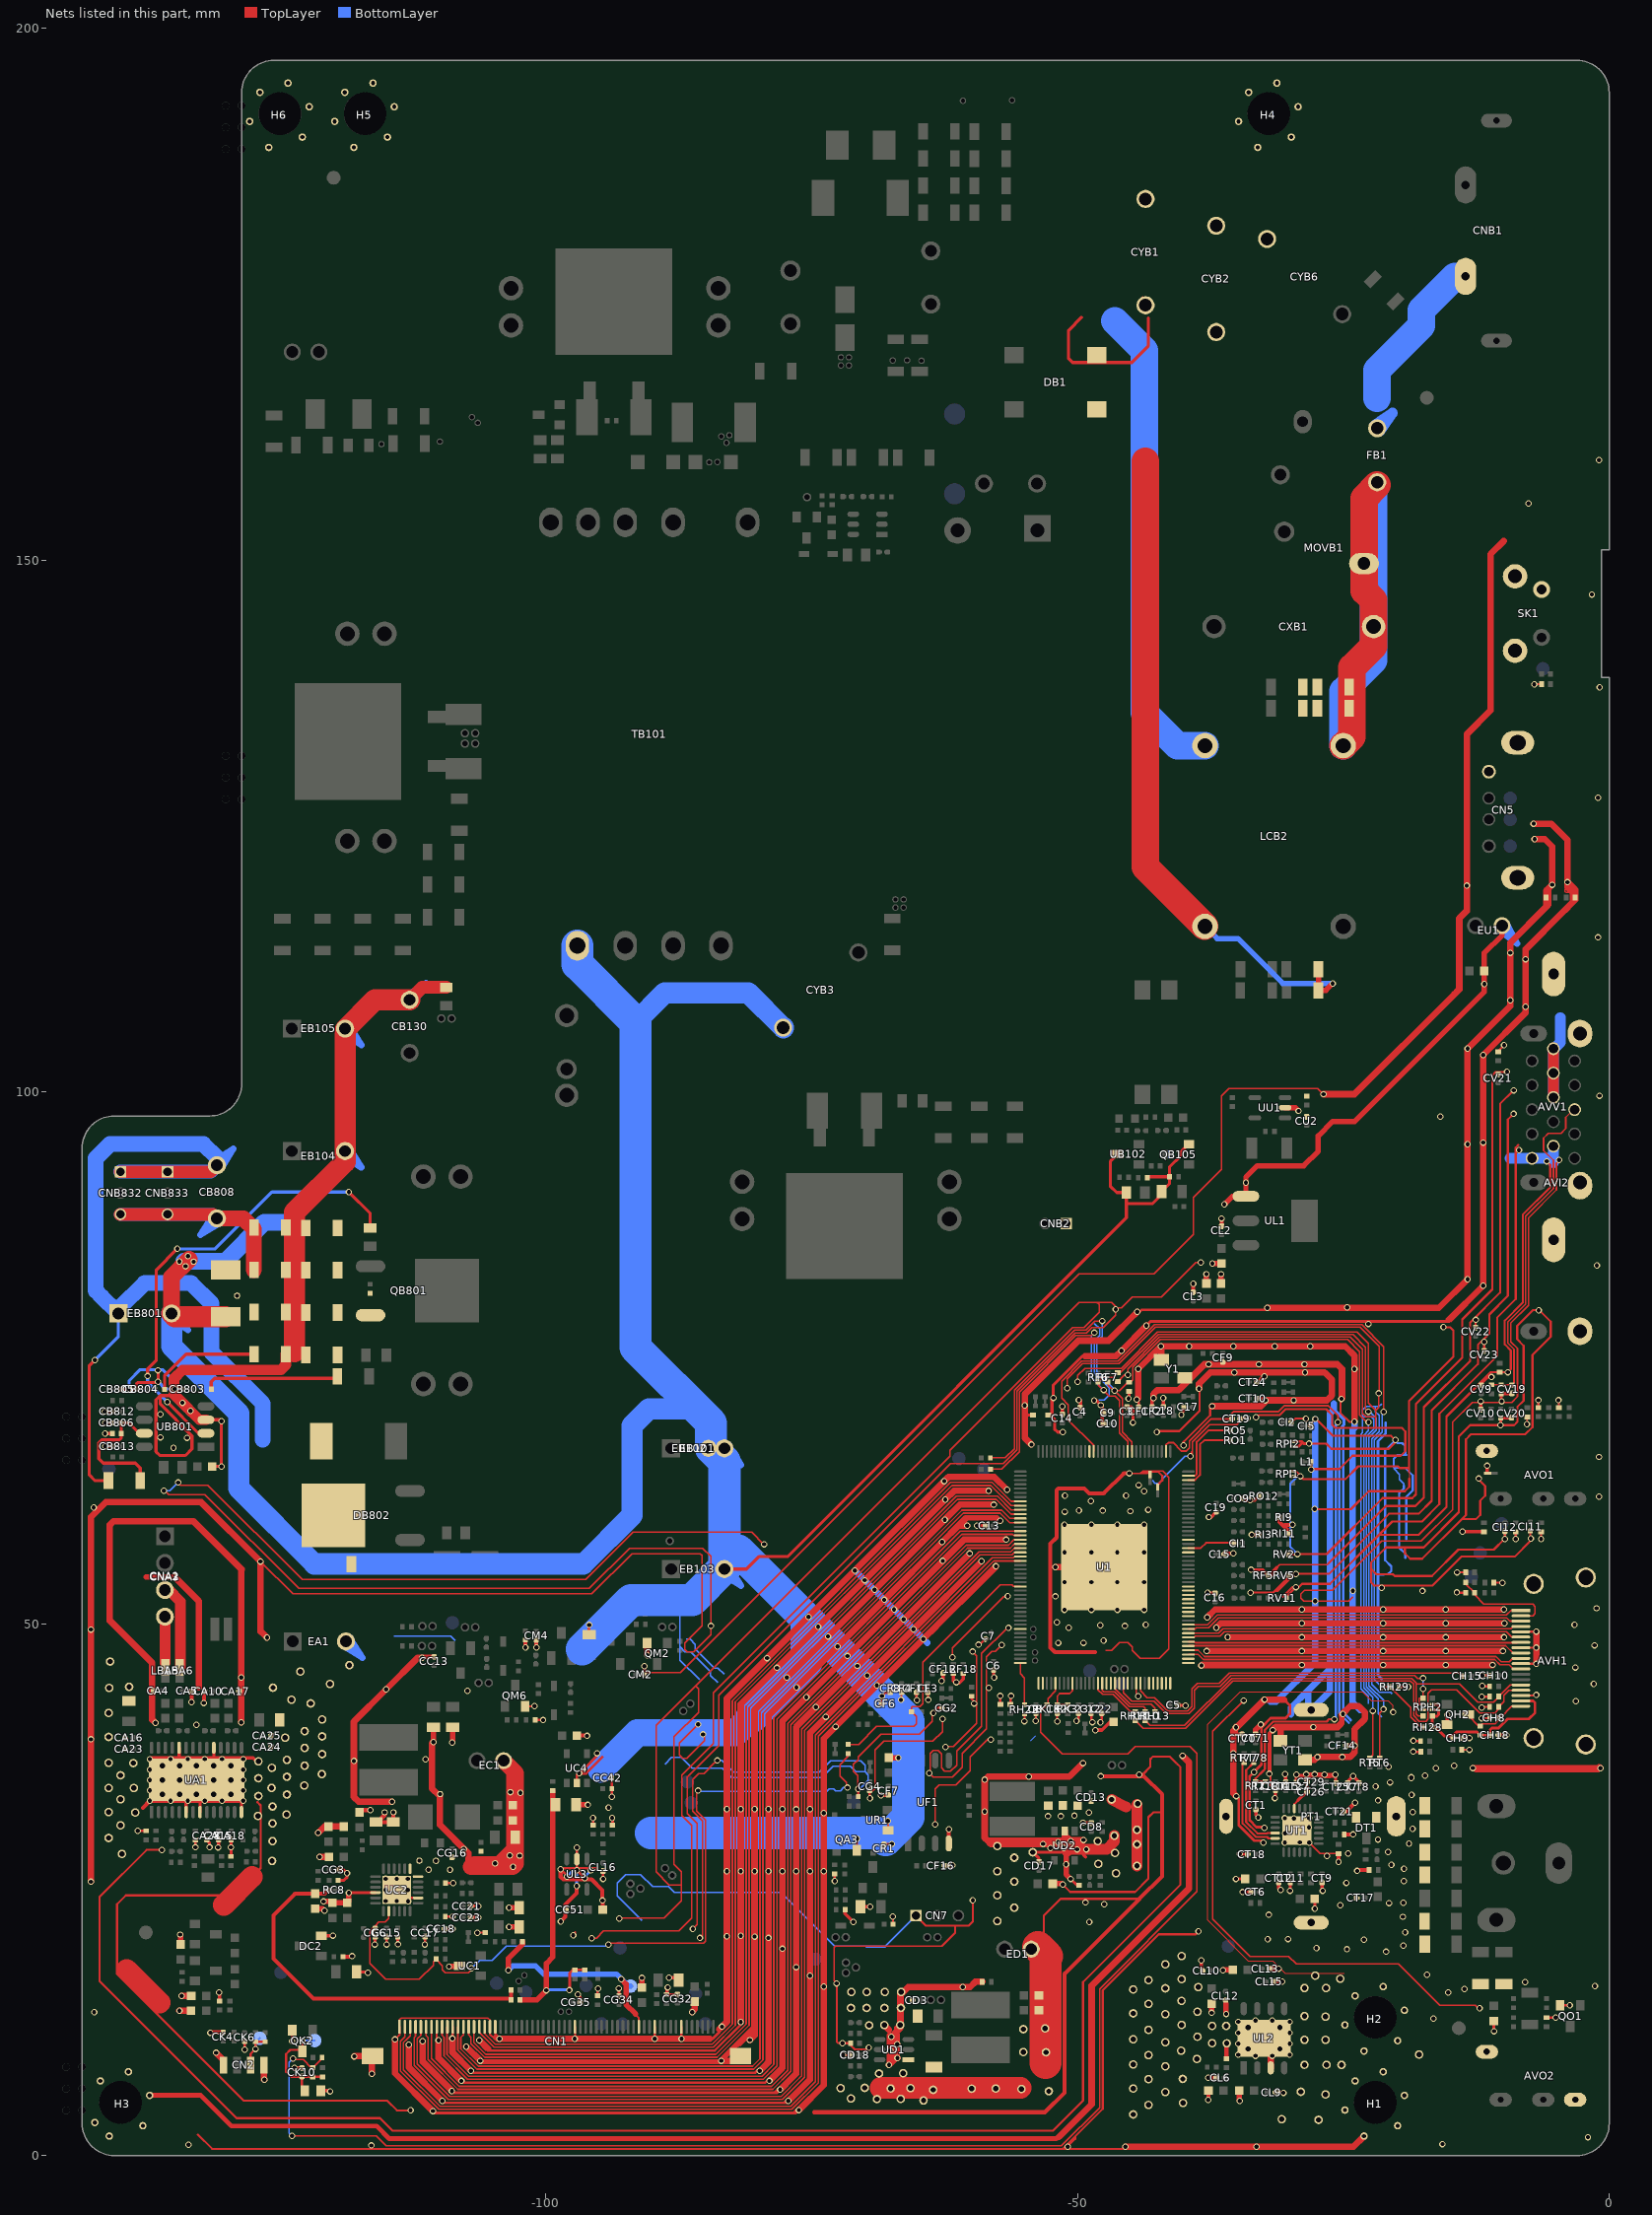
[diagram p0: the nets of this part, all layers, seen from the top]
# Altium PCB MISC86383-9.PcbDoc (part 12 of 18)
Units mm, origin at the board's own origin, x right, y up, seen from the top; angles counter-clockwise.
Board outline 143.6 x 197 mm, 2 copper layers (TopLayer, BottomLayer), stack 1.571 mm thick; 743 components, 401 nets, 2996 pads, 1077 vias.
Unrouted connection lines stored in the file: 4.

## Via types
v1: diameter 0.6, hole 0.4, TopLayer to BottomLayer, tented both sides, 993 vias
v2: diameter 0.6, hole 0.4, TopLayer to BottomLayer, 65 vias
v3: diameter 0.7, hole 0.5, TopLayer to BottomLayer, tented both sides, 15 vias
v4: diameter 0.8, hole 0.5, TopLayer to BottomLayer, tented both sides, 4 vias

## Nets (pads, with @x,y where several pads share a name; then routed paths per layer and width w, separated by ;. In a path a pad name is that pad's centre, name@x,y a point inside that pad or via, vN(x,y) a via of type N, cw(c..) or ccw(c..) an arc to the next point about the centre after c; other vN are vias at no path point) (continued)
GND: (continued)
  other v1: -116.412,0.947 -133.613,1.003 -15.673,1.074 -1.998,1.72 -33.252,9.371 -31.671,9.371 -34.884,9.476 -30.039,9.476 -34.884,10.508 -30.039,10.508 -34.884,11.539 -30.039,11.539 -34.884,12.571 -30.039,12.571 -33.252,12.677 -31.671,12.677 -16.523,12.874 -142.467,13.479 -15.146,15.329 -13.603,15.641 -1.344,15.939 -7.902,16.311 -17.141,16.988 -20.982,19.156 -24.662,19.388 -27.529,19.513 -19.363,19.748 -23.061,20.283 -32.119,20.335 -30.201,20.354 -19.19,20.979 -103.454,21.483 -48.895,21.971 -19.396,22.445 -32.013,22.636 -103.454,23.312 -47.498,23.622 -20.705,23.735 -49.258,23.792 -19.355,23.774 -112.943,23.91 -115.057,23.933 -114.012,23.927 -115.06,24.971 -112.968,24.975 -24.711,25.641 -19.317,25.819 -115.055,26.016 -114.016,26.02 -112.971,26.014 -82.969,26.73 -81.668,26.73 -80.368,26.738 -79.066,26.724 -77.765,26.736 -76.464,26.72 -75.164,26.732 -73.863,26.721 -19.293,26.964 -20.485,27.33 -25.448,27.612 -26.527,28.158 -24.559,28.399 -20.788,28.53 -52.527,28.905 -18.821,29.337 -30.509,29.42 -29.08,29.445 -21.742,29.719 -30.484,30.29 -28.235,30.85 -29.64,31.695 -30.509,31.72 -28.21,31.72 -52.781,31.902 -51.562,31.902 -50.292,31.953 -48.92,32.258 -18.476,32.296 -76.464,32.553 -81.668,32.563 -80.368,32.572 -79.066,32.557 -77.765,32.57 -75.164,32.565 -137.238,33.362 -135.287,33.368 -133.661,33.368 -132.061,33.368 -130.461,33.368 -21.739,33.39 -18.583,33.919 -137.238,34.339 -128.452,34.339 -21.968,34.717 -20.597,35.092 -137.238,35.316 -128.452,35.316 -18.607,35.499 -18.606,35.566 -17.324,35.719 -137.238,36.293 -128.452,36.293 -16.293,36.415 -20.736,36.565 -14.575,36.637 -111.316,37.254 -135.287,37.275 -133.661,37.275 -132.061,37.275 -130.461,37.275 -128.452,37.27 -35.343,37.81 -72.747,40.329 -132.85,40.498 -73.659,41.256 -74.587,42.167 -3.144,42.729 -75.495,43.098 -107.355,43.692 -76.424,44.01 -68.874,44.196 -1.445,44.34 -77.334,44.94 -69.785,45.124 -78.26,45.854 -3.173,45.892 -70.714,46.035 -79.18,46.773 -71.622,46.966 -72.55,47.877 -1.385,47.977 -51.816,48.209 -49.428,48.209 -47.549,48.412 -73.461,48.808 -50.815,49.641 -74.387,49.721 -45.532,49.793 -47.869,49.869 -43.576,49.895 -3.256,49.916 -51.932,50.141 -75.306,50.641 -51.221,51.313 -48.69,51.313 -46.252,51.313 -43.721,51.313 -21.26,51.337 -15.354,51.337 -1.181,51.458 -52.07,52.578 -24.105,53.102 -17.568,53.086 -51.221,53.916 -48.69,53.916 -46.252,53.916 -43.721,53.916 -126.835,55.854 -51.221,56.71 -48.69,56.71 -46.252,56.71 -43.721,56.71 -6.401,57.963 -51.221,59.313 -48.69,59.313 -46.252,59.313 -43.721,59.313 -51.196,60.537 -45.018,60.588 -47.634,60.639 -49.869,60.665 -43.343,60.723 -142.515,60.934 -48.741,61.548 -0.955,61.969 -45.43,62.036 -51.179,62.056 -43.726,62.471 -44.247,63.043 -0.91,99.652 -1.05,114.538 -1.045,127.688 -0.889,138.049 -1.626,146.787 -7.569,155.346 -0.947,159.42
  other v2: -135.014,66.535 -133.731,67.488 -136.233,67.539 -134.976,68.656 -136.246,69.698 -15.875,97.688
  other v3: -136.071,33.966 -134.445,33.966 -132.845,33.966 -131.245,33.966 -129.619,33.966 -136.071,35.316 -134.445,35.316 -131.245,35.316 -129.619,35.316 -136.071,36.666 -134.445,36.666 -132.845,36.666 -131.245,36.666 -129.619,36.666
  other v4: -33.961,10.024 -30.961,10.024 -33.961,12.024 -30.961,12.024
GND1: CYB1.2 CYB2.2 CYB6.2
GREF: CN1.46 GREF.1 RG48.2 | length 20.8
  TopLayer w0.203: -91.542,13.208 -91.25,12.916 CN1.46@-91.25,12.103
  TopLayer w0.508: v1(-103.518,17.424) -103.514,17.428 -103.514,18.535 -102.191,19.859 RG48.2@-102.191,20.117 ; v1(-92.9,16.586) -92.9,16.561 -92.456,16.116 -92.456,14.211 -91.542,13.297
  BottomLayer w0.508: v1(-103.518,17.424) -103.111,17.831 -100.97,17.831 -100.186,17.047 -93.361,17.047 v1(-92.9,16.586) -92.24,15.926 GREF.1@-92.024,15.926
GVOFF: CG6.1 RG49.1 RGV1.2 UC2.8 | length 74.4
  TopLayer w0.127: CG6.1@-116.046,21.38 -116.046,21.606 ; UC2.8@-114.764,22.973 -114.764,22.302 -115.123,21.943 -115.71,21.943 -116.046,21.606 ; v1(-106.985,17.59) -106.972,17.602 -106.883,17.602 -106.94,17.545 -107.281,17.204 -109.463,17.204 -109.73,17.471 -109.73,17.857 -110.305,18.432 RG49.1@-110.305,18.466 -110.579,18.192 -110.579,17.888 -111.894,16.573 -115.077,16.573 -116.566,18.062 -116.566,21.087 -116.16,21.493 -116.046,21.606 ; v1@-94.12,19.609 v1(-94.12,19.812) ; v1@-93.916,19.964 -85.166,19.964 -84.988,20.142 -84.988,31.556 -85.809,32.377 -85.809,34.193 v1(-85.687,34.315) ; v1(-71.628,34.595) -71.742,34.595 -71.742,35.056 -72.352,35.665 -72.352,36.747 -71.564,37.534 RGV1.2@-71.564,37.802
  BottomLayer w0.127: v1(-106.985,17.59) -106.223,18.351 -105.036,18.351 -103.715,19.672 -94.259,19.672 v1(-94.12,19.812) ; v1(-85.687,34.315) -85.598,34.227 -73.566,34.227 -73.33,34.463 -72.923,34.463 -72.75,34.29 -72.301,34.29 -71.996,34.595 v1(-71.628,34.595)
GVOFF/: RG40.1 RGV1.1 U1.106 | length 26.3
  TopLayer w0.127: RGV1.1@-71.564,38.652 -70.588,38.652 -68.888,40.352 -65.387,40.352 -65.168,40.571 -65.168,41.292 -65.601,41.725 RG40.1@-65.608,41.725 -65.608,42.113 -65.51,42.211 -64.799,42.211 -64.541,42.469 -64.541,46.391 -57.274,53.659 -56.147,53.659 -56.001,53.513 U1.106@-55.371,53.513
HD1_PB: U1.27
HD1_PR: U1.30
HD1_Y: CI1.1 U1.28 | length 4.5
  TopLayer w0.178: U1.28@-39.571,57.113 -38.404,57.113 -37.91,57.607 -35.343,57.607 CI1.1@-35.307,57.571
HDMI1_DET: U1.66
HDMI1_RX0_N: U1.153
HDMI1_RX0_P: U1.154
HDMI1_RX1_N: U1.155
HDMI1_RX1_P: U1.156
HDMI1_RX2_N: U1.1@-39.571,46.313 | length 0.3
  TopLayer w0.178: U1.1@-39.571,46.313 U1.1@-39.237,46.313
HDMI1_RX2_P: U1.2
HDMI1_RXC_N: U1.151
HDMI1_RXC_P: U1.152
HDMI1_SCL: U1.126
HDMI1_SDA: U1.125
HDMI2_5V: AVH1.18 CH9.2@-14.526,39.261 CH9.2@-14.701,39.261 CH18.2@-11.046,39.54 CH18.2@-11.221,39.54 RH14.2 RH28.2 RPH2.1 RPH2.3 RPH2.5 | length 17.7
  TopLayer w0.254: RPH2.3@-16.606,41.914 -16.146,41.914 -16.04,41.808 ; RPH2.5@-16.606,42.414 -16.602,42.418 -16.091,42.418 -16.04,42.367 -16.04,41.808 ; CH9.2@-14.783,39.439 -15.509,39.439 -16.354,40.284 RH28.2@-16.644,40.284 -16.644,41.276 RPH2.1@-16.606,41.314 -16.179,41.314 -16.04,41.453 -16.04,41.808 ; CH9.2@-14.701,39.261 -14.701,39.49 -14.371,39.82 -12.44,39.82 RH14.2@-12.142,39.522 -11.239,39.522 CH18.2@-11.221,39.54 -11.195,39.566 -11.195,40.029 -11.024,40.201 -10.412,40.201 -9.557,41.055 -7.56,41.055 -6.968,41.647 -6.968,42.57 -7.148,42.75 AVH1.18@-8.3,42.75
HDMI2_DET: RH28.1 RH29.1 U1.65 | length 79.6
  TopLayer w0.127: U1.65@-48.471,66.213 -48.471,66.759 -50.848,69.136 -50.848,70.584 -51.486,71.222 -51.486,72.805 -49.598,74.693 -46.197,74.693 -42.782,78.108 -23.269,78.108 -21.193,76.032 v1@-21.193,69.954 ; v1(-21.37,44.042) -21.351,44.061 RH29.1@-20.619,44.061 -18.656,42.098 -18.656,41.258 -17.682,40.284 RH28.1@-17.494,40.284
  BottomLayer w0.127: v1(-21.37,44.042) -22.068,44.74 -22.068,67.287 -21.331,68.024 v1@-21.331,69.803
  other v1: -21.216,69.93
HDMI2_RX0_N: AVH1.9 U1.5 | length 31.3
  TopLayer w0.155: U1.5@-39.571,47.913 -39.545,47.939 -9.732,47.939 -9.043,47.25 AVH1.9@-8.57,47.25
HDMI2_RX0_P: AVH1.7 U1.6 | length 31
  TopLayer w0.155: U1.6@-39.571,48.313 -38.991,48.313 -38.899,48.221 -8.64,48.221 AVH1.7@-8.611,48.25
HDMI2_RX1_N: AVH1.6 U1.7 | length 31.1
  TopLayer w0.155: U1.7@-39.571,48.713 -39.044,48.713 -38.949,48.808 -38.945,48.808 -38.922,48.831 -36.589,48.831 -36.175,49.246 -9.667,49.246 -9.171,48.75 AVH1.6@-8.926,48.75
HDMI2_RX1_P: AVH1.4@-8.3,49.75 U1.8 | length 31.5
  TopLayer w0.155: U1.8@-39.571,49.113 -36.732,49.113 -36.317,49.528 -9.245,49.528 -9.022,49.75 AVH1.4@-8.3,49.75
HDMI2_RX2_N: AVH1.3 U1.9 | length 31.8
  TopLayer w0.155: U1.9@-39.571,49.513 -38.93,49.513 -38.812,49.631 -37.654,49.631 -36.739,50.546 -9.642,50.546 -9.346,50.25 AVH1.3@-8.3,50.25
HDMI2_RX2_P: AVH1.1 U1.10 | length 31.3
  TopLayer w0.155: U1.10@-39.571,49.913 -37.771,49.913 -36.855,50.828 -9.655,50.828 -9.233,51.25 AVH1.1@-8.775,51.25
HDMI2_RXC_N: AVH1.12 U1.3 | length 31.8
  TopLayer w0.155: U1.3@-39.571,47.113 -38.653,47.113 -38.179,46.638 -10.759,46.638 -10.267,46.146 -9.418,46.146 -9.022,45.75 AVH1.12@-8.3,45.75
HDMI2_RXC_P: AVH1.10 U1.4 | length 31.9
  TopLayer w0.155: U1.4@-39.571,47.513 -38.654,47.513 -38.062,46.92 -10.643,46.92 -10.15,46.428 -9.397,46.428 -9.074,46.75 AVH1.10@-8.3,46.75
HDMI2_SCL: RH10.1 U1.140 | length 5.7
  TopLayer w0.127: U1.140@-47.671,44.413 -47.671,43.759 -47.515,43.603 -46.531,43.603 -45.128,42.2 -43.756,42.2 -43.635,42.079 RH10.1@-43.635,41.742
HDMI2_SCL/: AVH1.15 DH6.K RH10.2 RPH2.2 | length 42.6
  TopLayer w0.127: RH10.2@-43.635,40.892 -43.171,40.428 -39.931,40.428 -35.487,44.872 -18.579,44.872 -18.148,44.441 -18.148,44.342 ; RPH2.2@-17.506,41.314 -17.946,41.314 -18.148,41.516 -18.148,44.342 ; AVH1.15@-8.3,44.25 -9.293,44.25 DH6.K@-10.396,43.147 -10.396,43.115 -10.864,42.647 -12.374,42.647 -14.087,44.361 -18.129,44.361 -18.148,44.342
HDMI2_SDA: RH11.1 U1.139 | length 5
  TopLayer w0.127: U1.139@-48.071,44.413 -48.071,43.8 -47.62,43.349 -46.637,43.349 -45.03,41.742 RH11.1@-44.552,41.742
HDMI2_SDA/: AVH1.16 DH7.K RH11.2 RPH2.4 | length 47.1
  TopLayer w0.127: RH11.2@-44.552,40.892 -43.834,40.174 -39.825,40.174 -35.382,44.618 -18.684,44.618 -18.402,44.336 -18.402,41.363 -17.882,40.843 -17.208,40.843 -17.178,40.874 ; RPH2.4@-17.506,41.914 -17.06,41.914 -17.056,41.91 ; -17.177,40.874 -17.065,40.985 ; -17.065,40.986 -17.056,40.996 -17.056,41.91 ; AVH1.16@-8.3,43.75 -9.434,43.75 -9.893,43.291 -9.893,42.685 DH7.K@-10.396,42.182 -10.396,41.976 -10.749,41.623 -12.175,41.623 -14.342,43.79 -16.73,43.79 -17.056,43.464 -17.056,41.91
HDMI3_DET: U1.116
HDMI3_RX0_N: U1.14
HDMI3_RX0_P: U1.15
HDMI3_RX1_N: U1.16
HDMI3_RX1_P: U1.17
HDMI3_RX2_N: U1.18
HDMI3_RX2_P: U1.19
HDMI3_RXC_N: U1.12
HDMI3_RXC_P: U1.13
HDMI3_SCL: U1.142
HDMI3_SDA: U1.141
HDMI-CEC: RH13.2 U1.143 | length 5.4
  TopLayer w0.127: U1.143@-46.471,44.413 -46.471,43.902 -45.023,42.454 -43.083,42.454 -42.714,42.085 RH13.2@-42.714,41.742
HDMI_ARC: CH15.2@-13.623,45.072 CH15.2@-13.798,45.072 U1.149 | length 34.4
  TopLayer w0.127: U1.149@-44.071,44.413 -44.071,43.673 -43.442,43.044 -42.77,43.044 -41.526,41.8 -39.637,41.8 -39.243,42.194 -39.243,43.866 -38.726,44.383 -36.694,44.383 -35.698,45.38 -14.106,45.38 CH15.2@-13.798,45.072
HDMI_PIN2: AVH1.2 DH2.K RH1.1 | length 9.8
  TopLayer w0.127: RH1.1@-13.499,53.882 -13.499,53.766 DH2.K@-12.649,52.916 -12.649,52.717 -11.798,51.867 -7.188,51.867 -6.96,51.638 -6.96,50.966 -7.175,50.75 AVH1.2@-8.3,50.75
HOTPLUG1': U1.144
HOTPLUG2: AVH1.19 CH8.2@-10.396,41.166 CH8.2@-10.571,41.166 QH2.C RH14.1 | length 6
  TopLayer w0.127: QH2.C@-13.259,41.458 -13.259,41.368 -12.262,40.372 RH14.1@-12.142,40.372 -11.932,40.582 -10.745,40.582 -10.396,40.93 CH8.2@-10.396,41.115 ; QH2.C@-13.032,41.463 QH2.C@-13.032,41.483 ; CH8.2@-10.396,41.166 -10.245,41.166 -9.161,42.25 AVH1.19@-8.604,42.25
HOTPLUG2': RPH2.6 RPH2.8 U1.145 | length 35.6
  TopLayer w0.127: U1.145@-45.671,44.413 -45.671,44.2 -45.669,44.199 -45.669,43.491 -44.886,42.708 -42.793,42.708 -41.631,41.546 -39.531,41.546 -38.989,42.088 -38.989,43.761 -38.621,44.129 -36.589,44.129 -35.593,45.126 -18.278,45.126 -18.021,44.869 -17.526,44.869 v1@-17.57,44.825 ; -17.797,42.418 -17.801,42.414 ; RPH2.6@-17.506,42.414 -17.801,42.414 ; v1(-17.488,43.866) -17.506,43.848 RPH2.8@-17.506,43.014 -17.803,43.014 -17.88,42.937 -17.88,42.493 -17.801,42.414
  BottomLayer w0.127: v1(-17.488,43.866) v1(-17.488,44.882)
HOTPLUG3': U1.146
HS_VGA: AVV1.13 CV19.2@-9.155,72.306 CV19.2@-9.155,72.481 RV4.1 RV6.1 | length 32.2
  TopLayer w0.152: RV6.1@-11.016,72.481 RV4.1@-10.153,72.481 CV19.2@-9.155,72.481 -8.947,72.689 -8.947,75.827 -9.516,76.397 -9.516,78.381 -7.849,80.048 -7.849,88.314 -5.245,90.917 -5.245,93.581 -6.165,94.501 -6.165,95.67 -5.715,96.12 -4.526,96.12 -4.083,96.564 -4.083,97.615 -3.297,98.4 AVV1.13@-3.247,98.45
HVAA: CC43.2 RC33.2 RC36.2 RG42.1 RG43.1 | length 27
  TopLayer w0.254: v1(-97.79,15.545) -97.761,15.515 -97.761,15.545 -97.761,17.149 -97.454,17.456 RG43.1@-97.257,17.456 RG42.1@-96.342,17.456
  TopLayer w0.508: RC33.2@-102.42,14.631 -100.851,14.631 v1(-99.946,15.535) -99.946,18.062 -99.365,18.644 -99.365,32.982 RC36.2@-99.365,34.284
  BottomLayer w0.254: v1@-99.716,15.596 -97.841,15.596 v1(-97.79,15.545)
HVAA/: CC5.1 RC8.1 RC32.2 RC33.1 | length 34.9
  TopLayer w0.381: RC8.1@-120.472,24.948 -120.795,24.626 CC5.1@-121.672,24.626 -123.585,24.626 -125.609,22.601 -125.609,18.51 -121.844,14.745 RC33.1@-103.378,14.745 ; RC33.1@-103.27,14.631 RC32.2@-103.27,15.545
IF_AGC: CT19.2@-35.51,69.27 CT19.2@-35.335,69.27 RT2.2 RT18.2 U1.48 | length 61.8
  TopLayer w0.178: U1.48@-41.671,66.213 -41.671,66.802 -41.438,67.035 -41.019,67.035 -40.245,66.26 -39.764,66.26 -39.47,66.554 -39.47,67.215 -37.415,69.27 CT19.2@-35.51,69.27 -35.491,69.289 -35.491,69.778 -35.331,69.938 -31.128,69.938 -30.572,70.494 -26.409,70.494 -25.51,69.594 v1(-25.51,68.952)
  TopLayer w0.203: -32.495,36.212 -33.258,35.449 RT2.2@-33.258,35.161 -32.356,35.161 RT18.2@-32.344,35.149 ; -32.495,36.212 -32.369,36.337 -32.369,40.007 -31.579,40.797 -26.568,40.797 -26.322,41.043 -25.86,41.043 v1(-25.839,41.022)
  BottomLayer w0.203: v1(-25.839,41.022) -25.862,41.045 -25.709,41.198 -25.709,68.753 v1(-25.51,68.952)
IFn: RT78.1 UT1.16 | length 9.1
  TopLayer w0.203: RT78.1@-33.419,36.959 -34.135,36.242 -34.135,31.346 -33.081,30.292 -32.166,30.292 -32.138,30.32 UT1.16@-31.41,30.32
IFp: RT77.1 UT1.17 | length 9.4
  TopLayer w0.203: RT77.1@-34.337,36.959 -34.474,36.823 -34.474,31.217 -33.218,29.961 -32.166,29.961 -32.025,29.82 UT1.17@-31.41,29.82
IR: CN2.3 IR.1 RK15.2 RK16.2 | length 4.5
  TopLayer w0.203: CN2.3@-127.765,8.505 -127.765,9.56 v1(-127.305,10.02) RK16.2@-127.305,10.7 RK15.2@-126.39,10.7
  BottomLayer w0.203: v1(-127.305,10.02) -127.305,10.625 IR.1@-126.905,11.025
KEY: CK2.1 RK3.1 U1.133 | length 4.2
  TopLayer w0.152: RK3.1@-50.862,42.403 -50.907,42.403 CK2.1@-51.903,42.403 -51.903,43.215 -51.678,43.44 -50.733,43.44 -50.471,43.702 U1.133@-50.471,44.413
L: CYB1.1 DB1.2 LCB2.3 | length 61.2
  TopLayer w0.3: -49.619,172.847 -50.838,171.628 -50.838,168.973 -50.457,168.592 -48.17,168.592 -44.895,168.592 -43.345,170.142 -43.345,172.771 ; CYB1.1@-43.84,174.676 CYB1.1@-43.536,174.371 ; CYB1.1@-43.599,173.981 CYB1.1@-43.256,174.324
  BottomLayer w2.6: -46.495,172.529 -43.701,169.735 -43.701,135.674 -40.606,132.579 LCB2.3@-38.009,132.579
L-1: CNB1.1@-13.5,176.7 FB1.1 | length 14.5
  BottomLayer w2.6: -21.819,165.252 -21.819,167.894 -17.666,172.047 -17.666,173.545 -14.503,176.708
L-2: CXB1.1 FB1.2 LCB2.2 MOVB1.1 RB1.1 RB2.1 | length 52
  TopLayer w2.6: LCB2.2@-25.009,132.579 -24.188,133.4 -24.188,136.08 -24.188,138.087 -24.188,139.909 -22.154,141.942 CXB1.1@-22.154,143.764 -22.154,146.237 -23.06,147.142 -23.06,155.829 FB1.2@-21.819,157.07
  BottomLayer w2.6: LCB2.2@-25.009,132.579 -25.009,137.716 -22.154,140.571 CXB1.1@-22.154,143.764 -22.154,156.628 FB1.2@-22.001,156.781
L-N: RB1.2 RB2.2 RB3.1 RB4.1
LED+: CB808.2 CNB832.1 CNB833.1 DB801.K DB802.2 EB801.1@-140.193,79.184 RB812.2 RB814.1 | length 91.5
  TopLayer w0.3: v2(-142.405,74.803) -142.929,74.279 -142.929,63.995 -142.396,63.462 RB814.1@-141.137,63.462
  TopLayer w1.2: CNB832.1@-140,92.5 -131.539,92.5 CB808.2@-130.924,93.115
  BottomLayer w0.3: v2(-142.405,74.803) -140.193,77.015 EB801.1@-140.193,79.184
  BottomLayer w1.3: CNB832.1@-140,92.5 CNB833.1@-135.57,92.5 -131.539,92.5 CB808.2@-130.924,93.115
  BottomLayer w1.5: CB808.2@-130.924,93.115 -130.924,93.698 -130.924,93.84 -132.194,95.11 -140.995,95.11 -142.329,93.776 -142.329,81.32 -141.749,80.74 -140.373,79.364 EB801.1@-140.193,79.184 -140.193,79.567 -140.07,79.691 -137.719,82.042 -133.363,82.042 -131.445,80.124 -131.445,75.534 -126.617,70.706 -126.617,67.297
LED_CS: QB801.S RB806.2 RB808.1 RB810.2 RB818.1 RB819.1 RB820.1 RB821.1 | length 12.7
  TopLayer w0.3: RB806.2@-131.458,72.074 -131.458,72.771 -131.155,73.074 -119.803,73.074 RB810.2@-119.61,73.266
LED_FB: CB808.1 CNB832.3 CNB833.3 DB804.A pad.VIA5@-129.032,80.848 RB805.2 RB837.2 RB838.2 RB839.1 RB840.2 | length 36.7
  TopLayer w0.3: RB805.2@-135.853,72.038 -135.853,73.316 -133.82,75.349 RB839.1@-127.446,75.349
  TopLayer w1.2: CNB832.3@-140,88.5 -131.31,88.5 CB808.1@-130.924,88.114
  TopLayer w1.5: CB808.1@-130.924,88.114 -128.437,88.114 -127.446,87.123 RB837.2@-127.446,83.282
  BottomLayer w1.2: CNB832.3@-140,88.5 -131.31,88.5 CB808.1@-130.924,88.114
LED_GATE: RB807.1 UB801.2 | length 43.8
  TopLayer w0.3: v2(-137.452,73.292) -137.452,73.977 -136.627,74.803 -136.627,83.274 v2(-134.645,85.255) ; v2(-135.598,70.841) -132.668,67.91 UB801.2@-131.961,67.91 ; v2(-118.516,90.589) -116.523,88.595 RB807.1@-116.523,87.226
  BottomLayer w0.3: v2(-137.452,73.292) -137.452,72.695 v2(-135.598,70.841) v2@-135.547,70.891 ; v2(-134.645,85.255) -131.089,85.255 -125.755,90.589 v2(-118.516,90.589)
LED_OVP: CB806.1 RB803.2 RB814.2 UB801.7 | length 13.5
  TopLayer w0.3: RB803.2@-139.92,67.674 RB803.2@-139.92,67.894 ; RB814.2@-138.136,63.691 RB814.2@-138.136,63.906 ; RB814.2@-138.136,64.184 RB814.2@-138.136,63.906 ; UB801.7@-137.761,67.91 -138.243,67.91 -139.217,68.885 CB806.1@-139.92,68.885 RB803.2@-139.92,67.894 ; RB803.2@-139.92,67.894 -139.92,67.484 -140.119,67.285 -141.757,67.285 -142.03,67.012 -142.03,65.512 -141.633,65.115 -138.61,65.115 -138.136,64.642 RB814.2@-138.136,63.906
LED_R: CK10.2@-122.936,7.398 CK10.2@-122.936,7.573 DK20.A LED.1 QK2.C RK1.1 RK21.2 | length 10.6
  TopLayer w0.203: v1(-122.911,10.808) -122.911,10.668 -122.898,10.655 QK2.C@-122.898,9.804 -123.026,9.931 -124.028,9.931 -124.425,9.535 -124.425,7.877 -123.946,7.398 CK10.2@-122.936,7.398 ; DK20.A@-122.655,6.094 -122.936,6.375 CK10.2@-122.936,7.398 ; RK1.1@-121.006,7.398 RK21.2@-121.92,7.398 CK10.2@-122.936,7.398
  BottomLayer w0.203: v1(-122.911,10.808) LED.1@-121.729,10.808
LED_RED: RK18.1 RK20.2 RK21.1 U1.129 | length 147.4
  TopLayer w0.127: v1(-123.876,1.854) -115.939,1.854 -115.004,0.919 -51.507,0.919 -47.922,4.503 -47.922,15.654 -38.754,24.822 -38.754,37.812 -39.415,38.472 -44.545,38.472 -45.256,37.761 -51.407,37.761 -53.444,39.798 -53.444,41.787 -52.881,42.35 RK18.1@-52.881,42.403 ; v1@-123.812,8.877 v1@-123.761,8.877 ; v1(-123.761,9.106) -123.761,9.017 -122.822,9.017 -122.053,8.248 RK21.1@-121.92,8.248 -121.038,9.13 RK20.2@-121.038,9.195 ; RK18.1@-52.779,42.297 -52.779,42.403 -52.779,42.968 -52.071,43.676 U1.129@-52.071,44.413
  BottomLayer w0.127: v1(-123.876,1.854) -124.138,2.116 -124.138,8.73 v1(-123.761,9.106)
LINE_L_OUT: RO1.1 U1.44 | length 7.4
  TopLayer w0.178: U1.44@-39.571,63.513 -38.939,63.513 -38.476,63.976 -38.476,66.846 -38.06,67.262 RO1.1@-35.599,67.262 RO1.1@-35.719,67.142
LINE_R_OUT: RO5.1 U1.45 | length 6.9
  TopLayer w0.178: -38.97,63.913 -38.78,64.103 -38.78,67.114 -37.706,68.189 RO5.1@-35.599,68.189
LOUT+: CNA1.4 CNA2.4 CNA3.4 LBA5.2 LBA5.3 | length 4.3
  TopLayer w1.016: CNA3.4@-135.814,50.635 -135.791,50.612 LBA5.2@-135.791,46.334
LOUT-: CNA1.3 CNA2.3 CNA3.3 LBA6.2 LBA6.3 | length 8.1
  TopLayer w1.016: CNA3.3@-135.814,53.155 -135.425,53.155 -134.353,52.083 LBA6.3@-134.353,45.873
M_SCL_IC: DT3.K RF6.1 RG60.1 RT6.2 U1.57 | length 101.4
  TopLayer w0.127: RG60.1@-58.185,64.529 -57.112,64.529 -55.461,66.18 -55.461,71.782 -50.153,77.091 ; v1(-48.425,77.368) -48.677,77.116 ; RF6.1@-48.062,72.743 -48.062,72.45 -47.561,71.949 -47.033,71.421 -46.468,71.421 -46.032,70.984 -46.032,67.92 -45.271,67.159 U1.57@-45.271,66.213 ; RF6.1@-48.024,72.75 -47.615,73.159 -46.672,73.159 DT3.K@-46.235,73.596 ; DT3.K@-46.215,73.615 -45.948,73.615 -42.37,77.193 -24.094,77.193 -22.906,76.005 -22.906,70.21 v1(-22.639,69.943) ; RT6.2@-21.581,37.371 -21.581,41.605 v1(-21.224,41.963) ; -50.153,77.091 -48.703,77.091 -48.677,77.116 ; -50.153,77.091 -50.127,77.116 -48.677,77.116
  BottomLayer w0.127: v1(-48.425,77.368) -48.689,77.104 -48.689,73.155 v1(-47.522,71.988) ; v1(-22.639,69.943) -22.501,69.943 -21.882,69.324 -21.882,68.191 -22.576,67.497 -22.576,44.178 -21.224,42.826 v1(-21.224,41.963)
M_SDA_IC: DT2.K RF7.1 RG61.1 RT5.2 U1.56 | length 99.3
  TopLayer w0.127: RG61.1@-58.198,65.595 -56.787,65.595 -55.918,66.465 -55.918,71.972 -50.266,77.624 -49.222,77.624 -48.373,78.473 v1(-47.663,78.473) ; RF7.1@-47.109,72.743 -47.109,72.414 v1@-46.644,71.949 ; DT2.K@-45.148,72.597 DT2.K@-45.148,72.713 -45.257,72.713 -46.059,71.912 v1(-46.518,71.912) -45.778,71.171 -45.778,68.025 -44.871,67.118 U1.56@-44.871,66.213 ; DT2.K@-45.083,72.648 -44.789,72.942 -44.789,74.127 -42.18,76.736 -24.602,76.736 -23.465,75.598 -23.465,69.635 v1@-22.783,68.952 ; RT5.2@-22.496,37.371 -22.22,37.647 v1(-22.22,41.816)
  BottomLayer w0.127: v1(-47.663,78.473) -47.727,78.473 -47.695,78.442 -47.65,78.397 -47.65,77.025 -48.181,76.495 -48.181,73.7 v1@-46.541,72.06 ; v1(-22.627,68.952) -22.627,68.165 -23.084,67.708 -23.084,43.968 -22.22,43.104 v1(-22.22,41.816)
MHL_DET: RH22.2 U1.124 | length 4.1
  TopLayer w0.127: U1.124@-55.371,46.313 -55.371,45.306 -54.976,44.911 RH22.2@-54.976,42.365
MLV0N: CN1.3 U1.99 | length 104.2
  TopLayer w0.155: CN1.3@-112.75,12.103 -112.75,11.253 -113.08,10.923 -113.082,10.923 -113.381,10.625 -113.381,8.061 -109.938,4.619 -76.976,4.619 -74.654,6.94 -74.654,39.535 -57.994,56.195 -56.043,56.195 -55.925,56.313 U1.99@-55.371,56.313
MLV0P: CN1.2 U1.100 | length 104.6
  TopLayer w0.155: CN1.2@-113.25,12.103 -113.25,11.154 -113.662,10.742 -113.662,7.944 -110.055,4.337 -76.859,4.337 -74.372,6.823 -74.372,39.418 -57.878,55.913 U1.100@-55.371,55.913
MLV1N: CN1.5 U1.97 | length 102.1
  TopLayer w0.155: CN1.5@-111.75,12.103 -111.75,11.298 -112.08,10.968 -112.08,8.599 -109.044,5.563 -77.87,5.563 -76.104,7.329 -75.955,7.478 -75.955,14.122 -75.955,40.073 -59.27,56.759 -56.276,56.759 -55.922,57.113 U1.97@-55.371,57.113
MLV1P: CN1.4 U1.98 | length 102.4
  TopLayer w0.155: CN1.4@-112.25,12.103 -112.25,11.197 -112.362,11.085 -112.362,8.483 -109.161,5.281 -77.753,5.281 -75.673,7.362 -75.673,13.665 -75.673,39.956 -59.153,56.477 -56.16,56.477 -55.923,56.713 U1.98@-55.371,56.713
MLV2N: CN1.7 U1.95 | length 99.8
  TopLayer w0.155: CN1.7@-110.75,12.103 -110.75,9.109 -108.15,6.508 -78.764,6.508 -77.255,8.017 -77.255,13.614 -77.255,40.612 -60.47,57.397 -56.491,57.397 -55.976,57.913 U1.95@-55.371,57.913
MLV2P: CN1.6 U1.96 | length 100.3
  TopLayer w0.155: CN1.6@-111.25,12.103 -111.252,12.101 -111.252,11.278 -111.061,11.087 -111.061,9.021 -108.266,6.226 -78.647,6.226 -76.973,7.9 -76.973,13.056 -76.973,40.495 -60.353,57.115 -56.319,57.115 -55.921,57.513 U1.96@-55.371,57.513
MLV3N: CN1.13 U1.90 | length 96.5
  TopLayer w0.155: CN1.13@-107.75,12.103 -107.75,11.354 -107.992,11.112 -107.992,10.029 -106.361,8.398 -80.553,8.398 -79.857,9.094 -79.857,41.689 -60.861,60.685 -57.135,60.685 -56.362,59.913 U1.90@-55.371,59.913
MLV3P: CN1.12 U1.91 | length 97.6
  TopLayer w0.155: CN1.12@-108.25,12.103 -108.274,12.079 -108.274,9.912 -106.478,8.116 -80.436,8.116 -79.575,8.977 -79.575,22.882 ; -79.575,23.549 -79.575,22.882 ; U1.91@-55.371,59.513 -56.361,59.513 -57.251,60.403 -60.744,60.403 -79.575,41.573 -79.575,22.882
MLV4N: CN1.15 U1.88 | length 93.1
  TopLayer w0.155: CN1.15@-106.75,12.103 -106.75,10.626 -105.643,9.519 -84.004,9.519 -81.159,12.364 -81.159,12.845 -81.159,42.229 -61.4,61.987 -57.524,61.987 -56.25,60.713 U1.88@-55.371,60.713
MLV4P: CN1.14 U1.89 | length 93.7
  TopLayer w0.155: CN1.14@-107.25,12.103 -107.25,11.343 -107.032,11.125 -107.032,10.509 -105.759,9.237 -83.887,9.237 -80.877,12.247 -80.877,12.728 -80.877,12.845 -80.877,42.112 -61.284,61.705 -57.641,61.705 -56.249,60.313 U1.89@-55.371,60.313
MLV5N: CN1.17 U1.86 | length 91.9
  TopLayer w0.155: CN1.17@-105.75,12.103 -105.75,11.465 -104.748,10.464 -84.359,10.464 -82.459,12.364 -82.459,42.767 -61.939,63.288 -58.027,63.288 -56.253,61.513 U1.86@-55.371,61.513
MLV5P: CN1.16 U1.87 | length 92.5
  TopLayer w0.155: CN1.16@-106.25,12.103 -106.25,11.567 -104.865,10.182 -84.242,10.182 -82.177,12.247 -82.177,23.368 -82.177,42.651 -61.822,63.006 -58.144,63.006 -56.251,61.113 U1.87@-55.371,61.113
MLVCLKN: CN1.10 U1.93 | length 97.7
  TopLayer w0.155: CN1.10@-109.25,12.103 -109.292,12.06 -109.292,9.49 -107.255,7.453 -79.658,7.453 -78.556,8.556 -78.556,20.98 -78.556,41.151 -61.009,58.698 -55.499,58.698 -55.484,58.713 U1.93@-55.371,58.713
MLVCLKP: CN1.9 U1.94 | length 97.9
  TopLayer w0.155: CN1.9@-109.75,11.697 -109.75,11.291 -109.574,11.115 -109.574,9.373 -107.372,7.171 -79.542,7.171 -78.274,8.439 -78.274,23.266 -78.274,41.034 -60.892,58.416 -56.094,58.416 -55.991,58.313 U1.94@-55.371,58.313
N: CYB2.1 DB1.3 LCB2.4 RB101.1 RB141.2 | length 63.8
  TopLayer w0.5: RB141.2@-27.354,111.557 -27.342,111.544 RB101.1@-27.342,109.563 -26.645,109.563 v2(-25.997,110.211)
  TopLayer w2.6: -43.609,159.296 -43.609,121.179 LCB2.4@-38.047,115.617
  BottomLayer w0.5: LCB2.4@-38.009,115.579 -36.867,114.437 -34.924,114.437 -30.698,110.211 v2(-25.997,110.211)